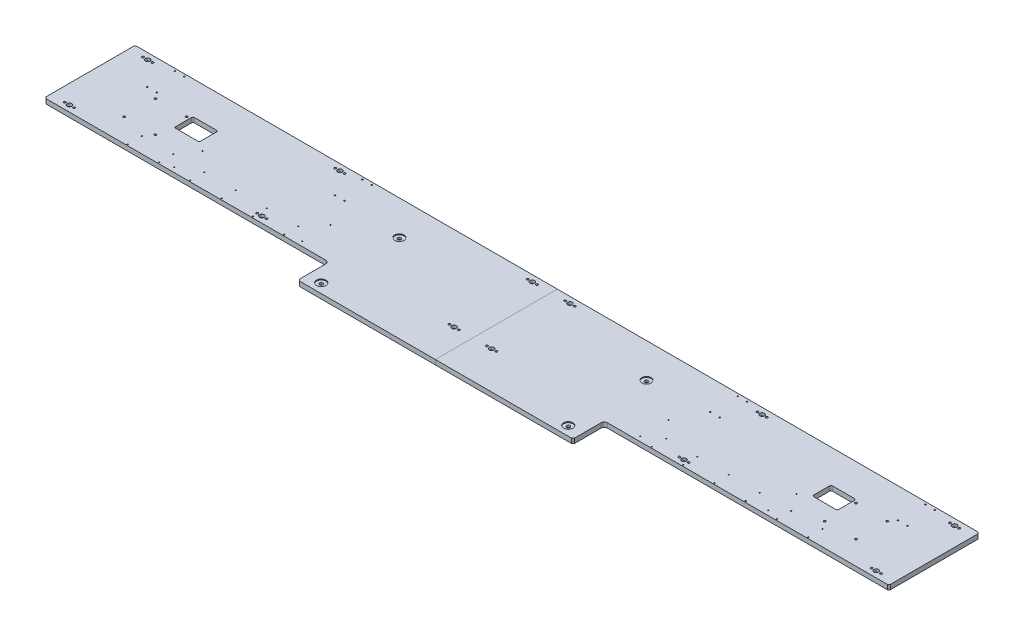
from build123d import *

# Parameters (mm, degrees)
SKETCH_1_W                = 2700
SKETCH_1_H                = 290
EXTRUDE_1_DEPTH           = 20
SKETCH_18_W               = 880
SKETCH_18_H               = 100
EXTRUDE_2_DEPTH           = 20
CHAMFER_1_SIZE            = 5
HOLE_WIZARD_1_D           = 9
HOLE_WIZARD_1_CBORE_D     = 15
HOLE_WIZARD_1_CBORE_DEPTH = 9
HOLE_WIZARD_M5_1_D        = 4.2
HOLE_WIZARD_M5_1_DEPTH    = 12.4
HOLE_WIZARD_M5_1_TIP      = 1.2618073
HOLE_WIZARD_M4_1_D        = 3.3
HOLE_WIZARD_M4_1_DEPTH    = 10.1
HOLE_WIZARD_M4_1_TIP      = 0.991420021
HOLE_WIZARD_M8_1_D        = 6.8
CUT_EXTRUDE_1_DEPTH       = 20
HOLE_WIZARD_3_D           = 11
HOLE_WIZARD_3_CBORE_D     = 18
HOLE_WIZARD_3_CBORE_DEPTH = 11
FILLET_1_R                = 10
HOLE_WIZARD_M8_2_D        = 6.8
SKETCH_21_R               = 15
CUT_EXTRUDE_2_DEPTH       = 3
HOLE_WIZARD_M4_2_D        = 3.3
SKETCH_25_W               = 3224.337080095
SKETCH_25_H               = 1222.940225485
CUT_EXTRUDE_3_DEPTH       = 5


with BuildPart() as part:
    # 草图1 → 凸台-拉伸1 (new body)
    with BuildSketch(Plane(origin=(0, 0, 0), x_dir=(1, 0, 0), z_dir=(0, 1, 0))):
        Rectangle(SKETCH_1_W, SKETCH_1_H)
    extrude(amount=EXTRUDE_1_DEPTH)

    # 草图18 → 凸台-拉伸2 (add)
    with BuildSketch(Plane(origin=(0, 20, 0), x_dir=(1, 0, 0), z_dir=(0, 1, 0))):
        with Locations((0, -195)):
            Rectangle(SKETCH_18_W, SKETCH_18_H)
    extrude(amount=-EXTRUDE_2_DEPTH)

    # 倒角1
    chamfer_1_edges = [part.edges().sort_by_distance(p)[0] for p in [
        (-440, 10, 245),
        (440, 10, 245),
        (1350, 10, 145),
        (-1350, 10, 145),
        (-1350, 10, -145),
        (1350, 10, -145),
    ]]
    chamfer(chamfer_1_edges, length=CHAMFER_1_SIZE)

    # 打孔尺寸(%根据)内六角圆柱头螺钉的类型1 (through all)
    with Locations(Plane(origin=(0, 20, 0), x_dir=(1, 0, 0), z_dir=(0, 1, 0))):
        with Locations((-1290, -125), (-675, -125), (-60, -125), (-675, 125), (-60, 125), (-1290, 125), (1290, 125), (60, 125), (675, 125), (60, -125), (675, -125), (1290, -125)):
            CounterBoreHole(HOLE_WIZARD_1_D / 2, HOLE_WIZARD_1_CBORE_D / 2, HOLE_WIZARD_1_CBORE_DEPTH)

    # M5 螺纹孔1
    with Locations(Plane(origin=(0, 20, 0), x_dir=(1, 0, 0), z_dir=(0, 1, 0))):
        with Locations((-585, 49.25), (-615, 49.25), (-1185, 49.25), (-1215, 49.25), (-585, 136.75), (-615, 136.75), (-1185, 136.75), (-1215, 136.75), (1215, 136.75), (1185, 136.75), (615, 136.75), (585, 136.75), (1215, 49.25), (1185, 49.25), (615, 49.25), (585, 49.25)):
            Hole(HOLE_WIZARD_M5_1_D / 2, depth=HOLE_WIZARD_M5_1_DEPTH)
            with Locations((0, 0, -(HOLE_WIZARD_M5_1_DEPTH + HOLE_WIZARD_M5_1_TIP / 2))):  # 118° drill point
                Cone(0, HOLE_WIZARD_M5_1_D / 2, HOLE_WIZARD_M5_1_TIP, mode=Mode.SUBTRACT)

    # M4 螺纹孔1
    with Locations(Plane(origin=(0, 20, 0), x_dir=(1, 0, 0), z_dir=(0, 1, 0))):
        with Locations((539.999999898, -40), (950, -129.999999534), (539.999999898, -129.999999534), (950, -40), (-950, -40), (-539.999999898, -129.999999534), (-950, -129.999999534), (-539.999999898, -40)):
            Hole(HOLE_WIZARD_M4_1_D / 2, depth=HOLE_WIZARD_M4_1_DEPTH)
            with Locations((0, 0, -(HOLE_WIZARD_M4_1_DEPTH + HOLE_WIZARD_M4_1_TIP / 2))):  # 118° drill point
                Cone(0, HOLE_WIZARD_M4_1_D / 2, HOLE_WIZARD_M4_1_TIP, mode=Mode.SUBTRACT)

    # M8 螺纹孔1 (through all)
    with Locations(Plane(origin=(0, 20, 0), x_dir=(1, 0, 0), z_dir=(0, 1, 0))):
        with Locations((-1305, -125), (-1275, -125), (-690, -125), (-660, -125), (-75, -125), (-45, -125), (-690, 125), (-660, 125), (-75, 125), (-45, 125), (-1305, 125), (-1275, 125), (1275, 125), (1305, 125), (45, 125), (75, 125), (660, 125), (690, 125), (45, -125), (75, -125), (660, -125), (690, -125), (1275, -125), (1305, -125)):
            Hole(HOLE_WIZARD_M8_1_D / 2)

    # 草图11 → 切除-拉伸1 (cut)
    with BuildSketch(Plane(origin=(0, 20, 0), x_dir=(1, 0, 0), z_dir=(0, 1, 0))):
        with BuildLine():
            Line((-1055, 40), (-985, 40))
            ThreePointArc((-985, 40), (-981.464466094, 38.535533906), (-980, 35))
            Line((-980, 35), (-980, -15))
            ThreePointArc((-980, -15), (-981.464466094, -18.535533906), (-985, -20))
            Line((-985, -20), (-1055, -20))
            ThreePointArc((-1055, -20), (-1058.535533906, -18.535533906), (-1060, -15))
            Line((-1060, -15), (-1060, 35))
            ThreePointArc((-1060, 35), (-1058.535533906, 38.535533906), (-1055, 40))
        make_face()
        with BuildLine():
            Line((980, 35), (980, -15))
            ThreePointArc((980, -15), (981.464466094, -18.535533906), (985, -20))
            Line((985, -20), (1055, -20))
            ThreePointArc((1055, -20), (1058.535533906, -18.535533906), (1060, -15))
            Line((1060, -15), (1060, 35))
            ThreePointArc((1060, 35), (1058.535533906, 38.535533906), (1055, 40))
            Line((1055, 40), (985, 40))
            ThreePointArc((985, 40), (981.464466094, 38.535533906), (980, 35))
        make_face()
    extrude(amount=-CUT_EXTRUDE_1_DEPTH, mode=Mode.SUBTRACT)

    # 打孔尺寸(%根据)内六角圆柱头螺钉的类型3 (through all)
    with Locations(Plane(origin=(0, 0, 0), x_dir=(-1, 0, 0), z_dir=(0, -1, 0))):
        with Locations((395, -215), (395, 35), (-395, 35), (-395, -215)):
            CounterBoreHole(HOLE_WIZARD_3_D / 2, HOLE_WIZARD_3_CBORE_D / 2, HOLE_WIZARD_3_CBORE_DEPTH)

    # 圆角1
    fillet_1_edges = [part.edges().sort_by_distance(p)[0] for p in [
        (-440, 10, 145),
        (440, 10, 145),
    ]]
    fillet(fillet_1_edges, radius=FILLET_1_R)

    # M8 螺纹孔2 (through all)
    with Locations(Plane(origin=(0, 20, 0), x_dir=(1, 0, 0), z_dir=(0, 1, 0))):
        with Locations((1170, 30), (1070, 30), (1070, -70), (1170, -70), (-1170, -70), (-1070, -70), (-1070, 30), (-1170, 30)):
            Hole(HOLE_WIZARD_M8_2_D / 2)

    # 草图21 → 切除-拉伸2 (cut)
    with BuildSketch(Plane.XZ.offset(-20)):
        with Locations(Location((395, 215, 0), (0, 0, 270))):
            Circle(SKETCH_21_R)
        with Locations(Location((395, -35, 0), (0, 0, 270))):
            Circle(SKETCH_21_R)
        with Locations(Location((-395, -35, 0), (0, 0, 90))):
            Circle(SKETCH_21_R)
        with Locations(Location((-395, 215, 0), (0, 0, 90))):
            Circle(SKETCH_21_R)
    extrude(amount=CUT_EXTRUDE_2_DEPTH, mode=Mode.SUBTRACT)

    # M4 螺纹孔2 (through all)
    with Locations(Plane(origin=(0, 20, 0), x_dir=(1, 0, 0), z_dir=(0, 1, 0))):
        with Locations((-1088, -95.5), (-1088, -140.5), (-988, -95.5), (-988, -140.5), (-888, -95.5), (-888, -140.5), (-788, -95.5), (-788, -140.5), (-688, -95.5), (-688, -140.5), (688, -140.5), (688, -95.5), (788, -140.5), (788, -95.5), (888, -140.5), (888, -95.5), (988, -140.5), (988, -95.5), (1088, -140.5), (1088, -95.5), (-588, -95.5), (-588, -140.5), (588, -140.5), (588, -95.5)):
            Hole(HOLE_WIZARD_M4_2_D / 2)

    # 草图25 → 切除-拉伸3 (cut)
    with BuildSketch(Plane.XZ):
        with Locations((-5.083862384, 31.100873151)):
            Rectangle(SKETCH_25_W, SKETCH_25_H)
    extrude(amount=-CUT_EXTRUDE_3_DEPTH, mode=Mode.SUBTRACT)


solid = part.part
